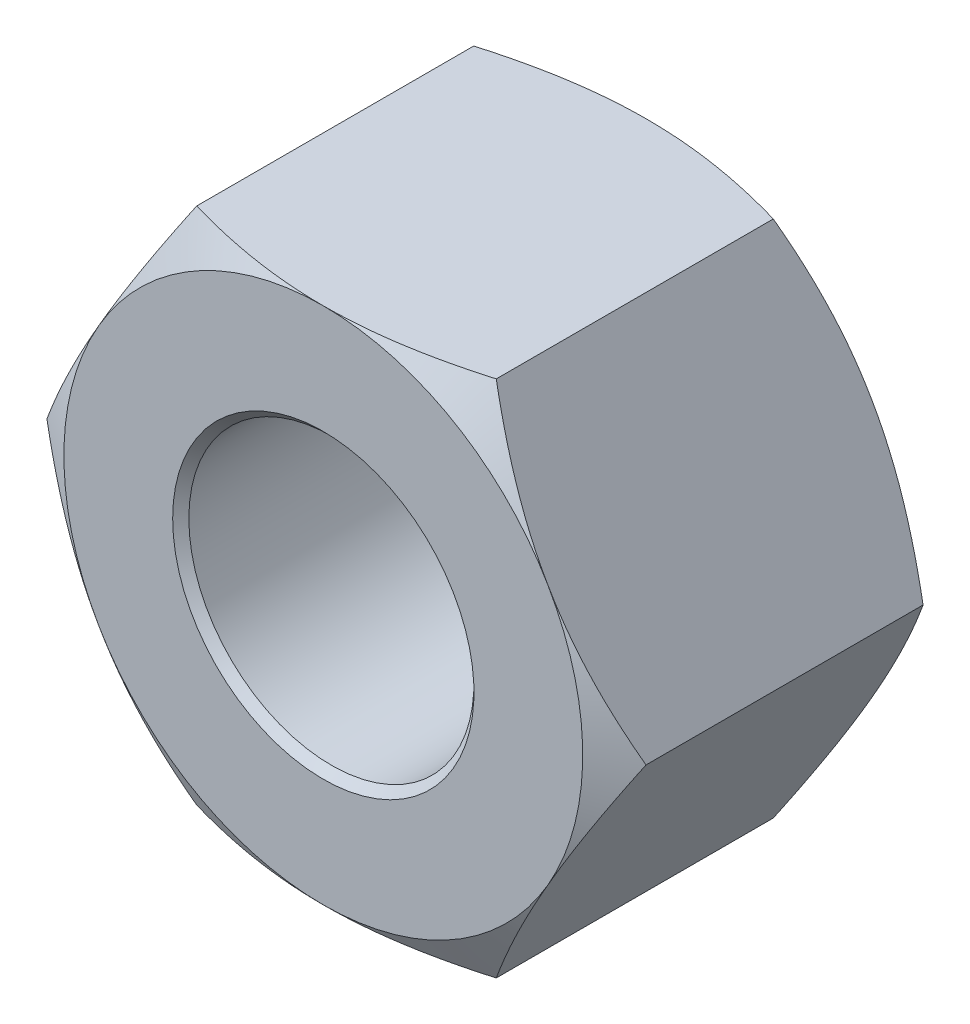
SolidWorks part; units mm, degrees
material "Q235"
ref_plane "Plane1" through (0, 0, 0) normal (0, 0, 1) x (1, 0, 0)
ref_plane "Plane2" through (0, 0, 0) normal (0, 1, 0) x (1, 0, 0)
ref_plane "Plane3" through (0, 0, 0) normal (1, 0, 0) x (0, 0, -1)
sketch "Dimension Sketch" plane through (0, 0, 0) normal (0, 0, 1) x (1, 0, 0)
  line L0 (0, 0) -> (16, 0) construction
  point P1 (14.5, 0)
  point P3 (10, 0)
  point P4 (1.5, 0)
  point P5 (17.6, 0)
  point P6 (9.5, 0)
  point P8 (16, 0)
  dimension "D" = 10
  dimension "e(最小)" = 17.6
  dimension "m(最大)" = 9.5
  dimension "s(公称)" = 16
  dimension "dw(最小)" = 14.5
  dimension "P" = 1.5
sketch "Sketch1" plane through (0, 0, 0) normal (0, 0, 1) x (1, 0, 0)
  line L0 (-26.8088, 0) -> (37.1748, 0) construction
  line L1 (0, 25.0215) -> (0, -25.0215) construction
  line L3 (4.4, 7.621) -> (-4.4, 7.621)
  line L4 (-4.4, 7.621) -> (-8.8, 0)
  line L5 (-8.8, 0) -> (-4.4, -7.621)
  line L6 (-4.4, -7.621) -> (4.4, -7.621)
  line L7 (4.4, -7.621) -> (8.8, 0)
  line L8 (8.8, 0) -> (4.4, 7.621)
  circle A0 centre (0, 0) radius 7.621 construction
  circle A1 centre (0, 0) radius 4.1881
  dimension "D" = 8.3763
  dimension "e" = 17.6
extrude "Boss-Extrude" add sketch "Sketch1" along normal blind 9.5
cosmetic thread "Cosmetic Thread1" parameters "D2"=10
sketch "Sketch2" plane through (0, 0, 0) normal (0, 0, -1) x (-1, 0, 0)
  line L0 (-4.4, 7.621) -> (4.4, 7.621) construction
  circle A0 centre (0, 0) radius 7.621
  circle A1 centre (0, 0) radius 4.1881 construction
extrude "Cut-Extrude1" cut sketch "Sketch2" against normal through all draft 60 flip side to cut
sketch "Sketch3" plane through (0, 0, 9.5) normal (0, 0, 1) x (1, 0, 0)
  line L0 (8.8, 0) -> (4.4, 7.621) construction
  circle A0 centre (0, 0) radius 7.621
extrude "Cut-Extrude2" cut sketch "Sketch3" against normal through all draft 60 flip side to cut
chamfer "Chamfer1" distance 0.2375 angle 45 2 edges at (4.1881, 0, 0) (4.1881, 0, 9.5)
